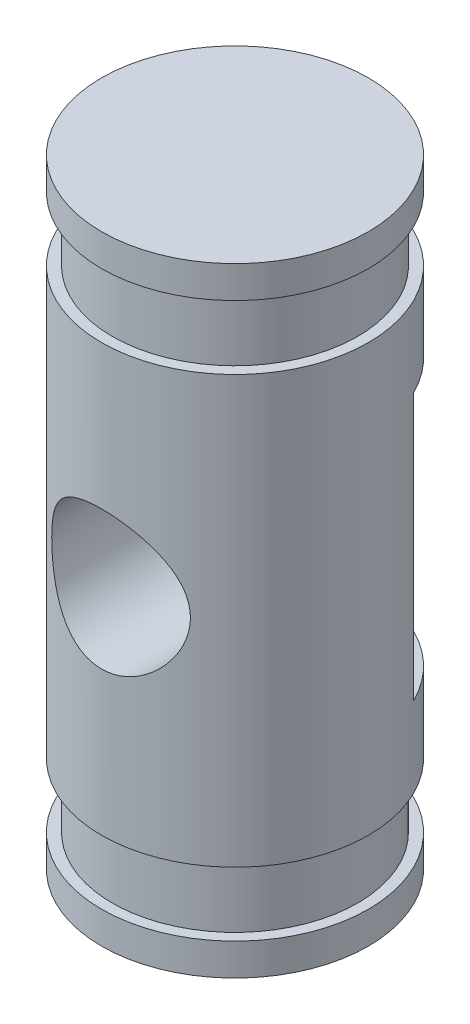
from build123d import *

# Parameters (mm, degrees)
SKETCH1_R           = 12.5
BOSS_EXTRUDE1_DEPTH = 29
CUT_EXTRUDE1_START  = -3
SKETCH2_R           = 12.5
SKETCH2_R_2         = 11.5
CUT_EXTRUDE1_DEPTH  = 6
SKETCH3_W           = 7
SKETCH3_H           = 25
CUT_EXTRUDE2_DEPTH  = 33
SKETCH4_R           = 6.5
CUT_EXTRUDE3_DEPTH  = 37.349002737


with BuildPart() as part:
    # Sketch1 → Boss-Extrude1 (new, symmetric)
    with BuildSketch(Plane(origin=(0, 0, 0), x_dir=(1, 0, 0), z_dir=(0, 1, 0))):
        with Locations(Location((0, 0, 0), (0, 0, 90))):
            Circle(SKETCH1_R)
    extrude(amount=BOSS_EXTRUDE1_DEPTH, both=True)

    # Sketch2 → Cut-Extrude1 (cut)
    with BuildSketch(Plane(origin=(0, 29, 0), x_dir=(1, 0, 0), z_dir=(0, 1, 0)).offset(CUT_EXTRUDE1_START)):
        with Locations(Location((0, 0, 0), (0, 0, 90))):
            Circle(SKETCH2_R)
        with Locations(Location((0, 0, 0), (0, 0, 270))):
            Circle(SKETCH2_R_2, mode=Mode.SUBTRACT)
    cut_extrude1 = extrude(amount=-CUT_EXTRUDE1_DEPTH, mode=Mode.SUBTRACT)

    # Mirror1: Cut-Extrude1 across plane
    add(cut_extrude1.mirror(Plane.ZX), mode=Mode.SUBTRACT)

    # Sketch3 → Cut-Extrude2 (cut, symmetric)
    with BuildSketch(Plane(origin=(0, 0, 0), x_dir=(0, 0, -1), z_dir=(1, 0, 0))):
        with Locations((9, 0)):
            Rectangle(SKETCH3_W, SKETCH3_H)
    extrude(amount=CUT_EXTRUDE2_DEPTH, both=True, mode=Mode.SUBTRACT)

    # Sketch4 → Cut-Extrude3 (cut, through all)
    with BuildSketch(Plane(origin=(0, 0, -5.5), x_dir=(-1, 0, 0), z_dir=(0, 0, -1))):
        with Locations(Location((0, 0, 0), (0, 0, 90))):
            Circle(SKETCH4_R)
    extrude(amount=-CUT_EXTRUDE3_DEPTH, mode=Mode.SUBTRACT)


solid = part.part
